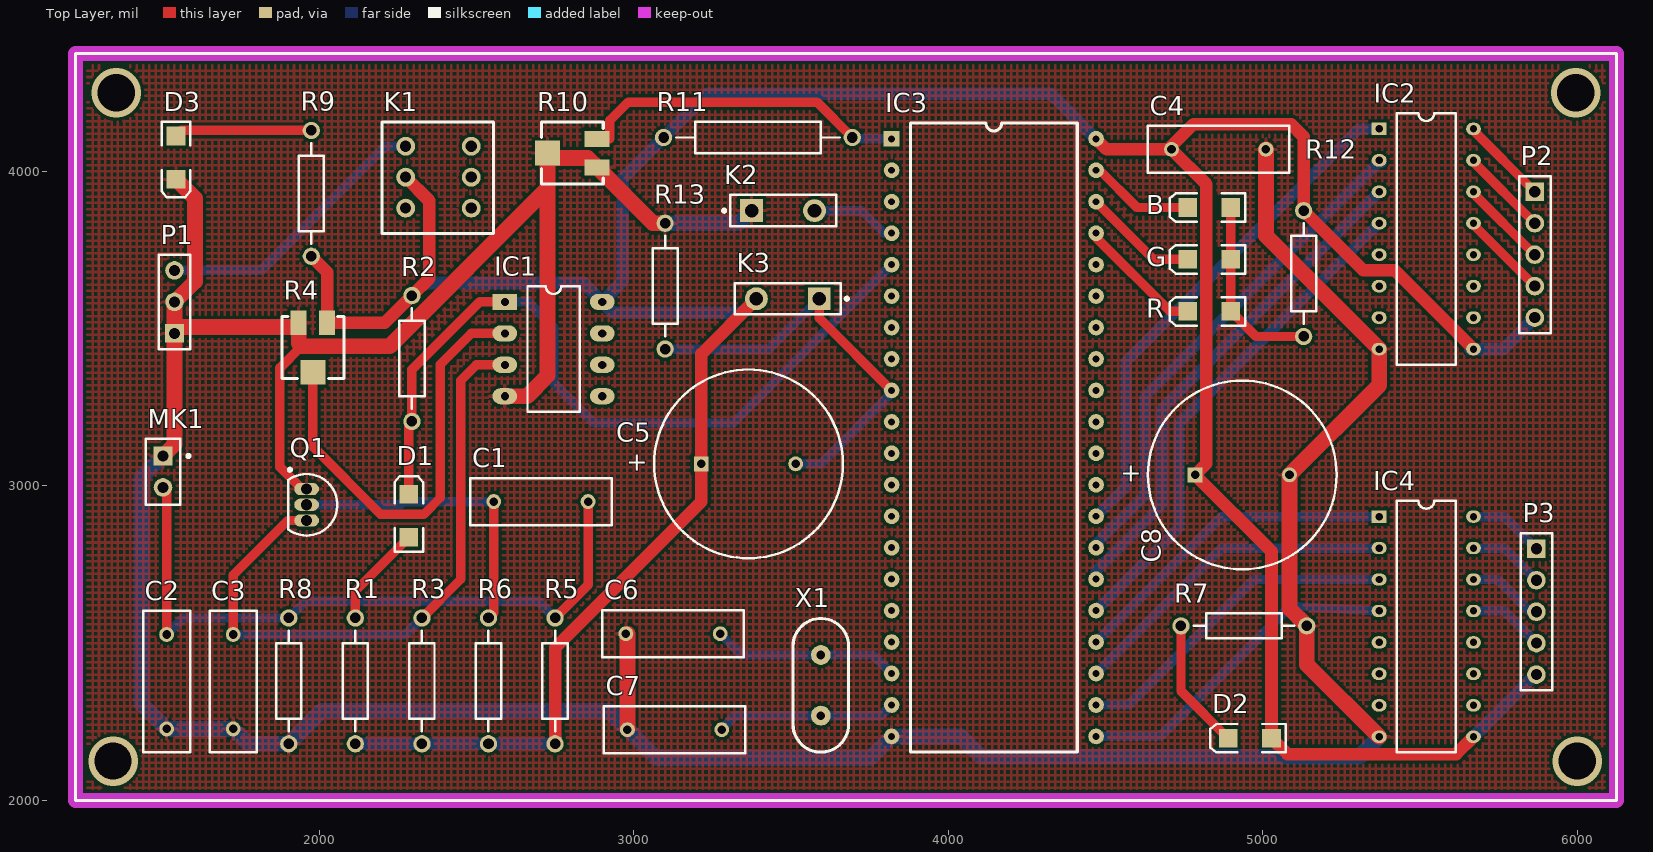
[diagram p0: Top Layer view]
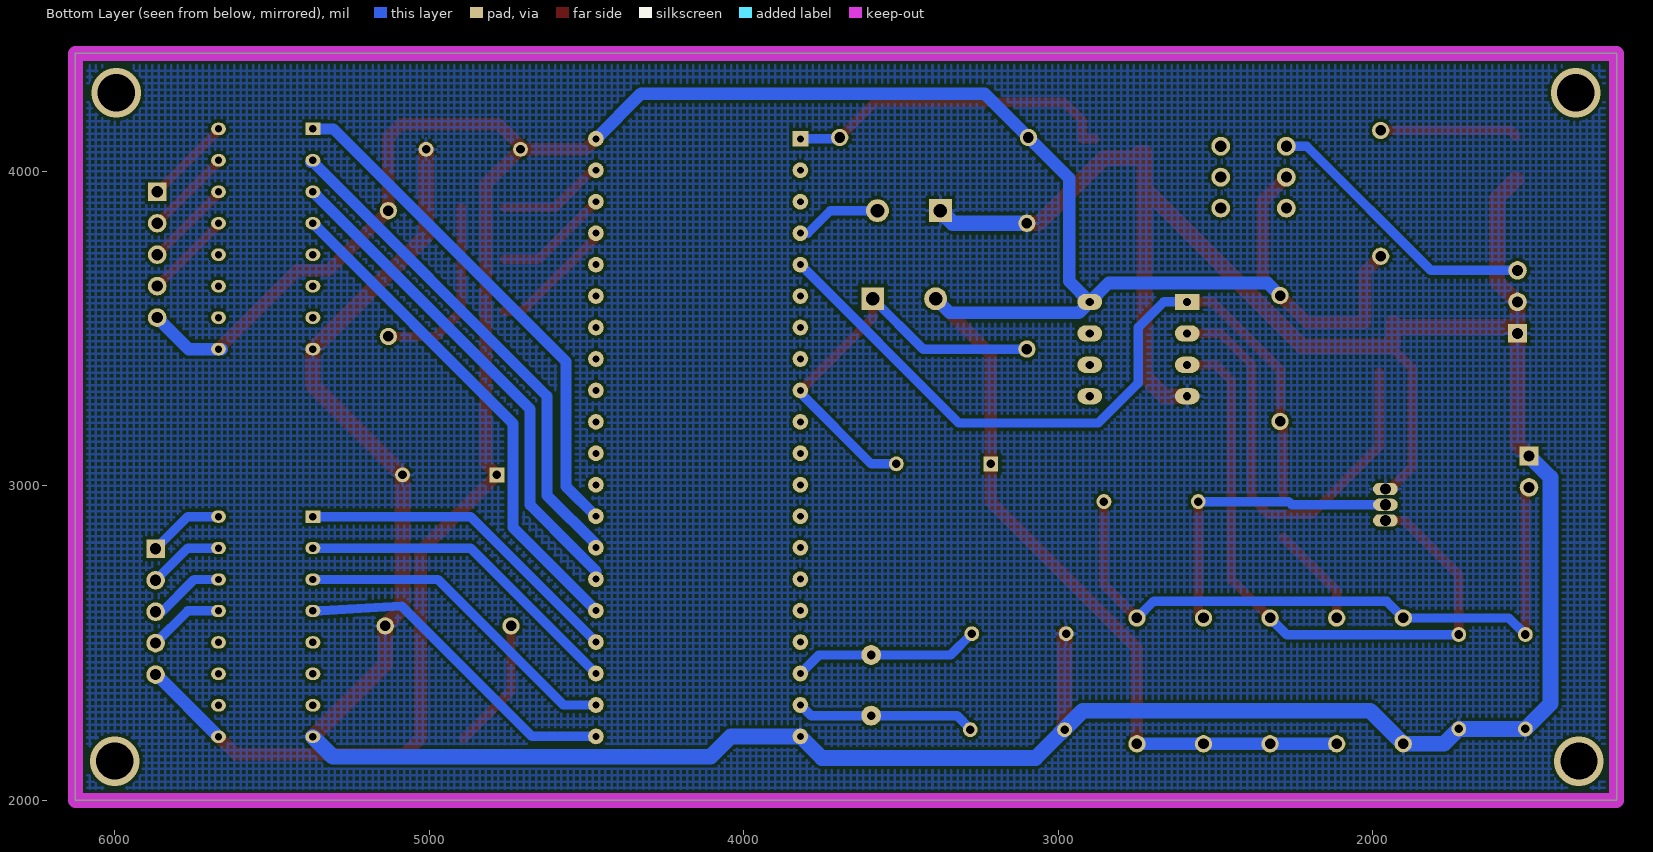
[diagram p1: Bottom Layer view, seen from below]
# Altium PCB MISC86340.PcbDoc
Units mil, origin at the board's own origin, x right, y up, seen from the top; angles counter-clockwise.
Board outline 4900 x 2375 mil, 2 copper layers (Top Layer, Bottom Layer); 40 components, 36 nets, 166 pads, 4 vias.

## Layer stack, top to bottom (the 12.6 mil dielectric is the usual default, probably not edited)
Top Solder: solder mask 0.4, Solder Resist, Dk 3.5
Top Layer: signal copper 1.4
Dielectric 1: dielectric 12.6, FR-4, Dk 4.8
Bottom Layer: signal copper 1.4
Bottom Solder: solder mask 0.4, Solder Resist, Dk 3.5

## Board outline
1225,2000 1225,4375 6125,4375 6125,2000

## Design rules (kind name [scope] priority, off if disabled: settings)
Clearance [All] p1: gap=10
HoleSize [All] p1: absolutevalues=TRUE maxlimit=500 minlimit=1 maxpercent=80.000 minpercent=20.000
MinimumSolderMaskSliver [All] p1: minsoldermaskwidth=2
PolygonConnect [All] p1: connectstyle=Relief reliefconductorwidth=10 reliefentries=4 polygonreliefangle="90 Angle" airgapwidth=10
RoomDefinition 声光控窗帘 [InComponentClass('声光控窗帘')] p1: confinementstyle=ConfineIn formatcopy=TRUE lockcomponents=FALSE outline 1205,1975 6145,1975 6145,4380 1205,4380
RoutingVias [All] p1: holewidth=28 width=50 viastyle="Through Hole" minholewidth=28 minwidth=50 maxholewidth=28 maxwidth=50
SilkToSilkClearance [All] p1: silktosilkclearance=2
SilkToSolderMaskClearance [IsPad] p1: minsilkscreentomaskgap=0 clearancetoexposedcopper=TRUE
SolderMaskExpansion [All] p1: expansion=4
Width GND [InNet('GND')] p1: maxlimit=55 minlimit=30 preferedwidth=50
Width VCC [InNet('VCC')] p2: maxlimit=45 minlimit=30 preferedwidth=40
Width [All] p3: maxlimit=35 minlimit=20 preferedwidth=30
26 further rules are at their usual default settings.

## Components (designator, comment, footprint, x,y, rotation, side; value= is the part's Value field where it differs from the comment)
B "LED2" 3.2X1.6X1.1 4830,3885 r180 top
C1 "Cap" RAD-0.3 2705,2950 r180 top
C2 "Cap" RAD-0.3 1515,2377.38 r270 top
C3 "Cap" RAD-0.3 1726.67,2377.38 r270 top
C4 "Cap" RAD-0.3 4860,4070 r0 top
C5 "Cap Pol1" RB7.6-15 3365,3070 r180 top
C6 "Cap" RAD-0.3 3125,2530 r180 top
C7 "Cap" RAD-0.3 3130,2225 r180 top
C8 "Cap Pol1" RB7.6-15 4935,3035 r180 top
D1 "LED2" 3.2X1.6X1.1 2285,2905 r90 top
D2 "LED2" 3.2X1.6X1.1 4958.9,2197.65 r180 top
D3 "LED2" 3.2X1.6X1.1 1544.72,4043.45 r270 top
G "LED2" 3.2X1.6X1.1 4830,3720 r180 top
IC1 "LM393" LM393 2590.16,3585 r0 top
IC2 "ULN2003" ULN2003 5370,4135 r0 top
IC3 "89c51" 89c51 3820,4103.44 r0 top
IC4 "ULN2003" ULN2003 5370,2902.38 r0 top
K1 "Component_1" 自锁开关 2200,4156.56 r270 top
K2 "SW-PB" SPST-2 3475,3875 r0 top
K3 "SW-PB" SPST-2 3490,3595 r180 top
MK1 "Mic2" PIN2 1503.39,3095 r270 top
P1 "Header 3" HDR1X3 1540,3485 r90 top
P2 "Header 5" HDR1X5 5865,3935 r270 top
P3 "Header 5" HDR1X5 5870,2800 r270 top
Q1 "2N3904" TO-92A 1960,2940 r180 top
R "LED2" 3.2X1.6X1.1 4830,3555 r180 top
R1 "Res2" AXIAL-0.4 2115,2380 r90 top
R2 "Res2" AXIAL-0.4 2295,3405 r270 top
R3 "Res2" AXIAL-0.4 2326.67,2380 r270 top
R4 "RPot SM" POT4MM-2 1980,3440 r270 top
R5 "Res2" AXIAL-0.4 2750,2380 r270 top
R6 "Res2" AXIAL-0.4 2538.33,2380 r270 top
R7 "Res2" AXIAL-0.4 4940,2555 r180 top
R8 "Res2" AXIAL-0.4 1903.33,2380 r90 top
R9 "Res2" AXIAL-0.4 1975,3930 r90 top
R10 "RPot SM" POT4MM-2 2805,4058.13 r180 top
R11 "Res Adj2" AXIAL-0.6 3395,4107.62 r180 top
R12 "Res2" AXIAL-0.4 5130,3675 r270 top
R13 "Res2" AXIAL-0.4 3100,3635 r90 top
X1 "Component_1" LC-HC-49S 3595,2365.94 r90 top

## Footprints (in the part's own frame and the unit in brackets; to place one, negate y for a bottom-side part, rotate by r counter-clockwise, add the part's x,y. Pads: shape width x height; smd on the part's side, far side on the other; paste and mask are expansions set on the pad)
3.2X1.6X1.1 [mm] "SMT LED; 2 Flat Leads"
  rect 1.5x1.5 smd: 1(-1.75,0) 2(1.75,0)
  silkscreen extent -2.9,-1.15 3.2,1.15
89c51 [mil]
  rect 50x50 hole 22: 1(0,0)
  round 50 hole 22: 2(0,-100) 3(0,-200) 4(0,-300) 5(0,-400) 6(0,-500) 7(0,-600) 8(0,-700) 9(0,-800) 10(0,-900) 11(0,-1000) 12(0,-1100) 13(0,-1200) 14(0,-1300) 15(0,-1400) 16(0,-1500) 17(0,-1600) 18(0,-1700) 19(0,-1800) 20(0,-1900) 21(650,-1900) 22(650,-1800) 23(650,-1700) 24(650,-1600) 25(650,-1500) 26(650,-1400) 27(650,-1300) 28(650,-1200) 29(650,-1100) 30(650,-1000) 31(650,-900) 32(650,-800) 33(650,-700) 34(650,-600) 35(650,-500) 36(650,-400) 37(650,-300) 38(650,-200) 39(650,-100) 40(650,0)
  silkscreen extent 60,-1950 590,50, body extent 65,-1950 590,55, height 190
AXIAL-0.4 [mm] "Axial Device, Thru-Hole; 2 Leads; 0.4 in Pin Spacing"
  round 1.4 hole 0.85: 1(-5.08,0) 2(5.08,0)
  silkscreen extent -4.06,-1.02 4.06,1.02
AXIAL-0.6 [mm] "Axial Device, Thru-Hole; 2 Leads; 0.6 in Pin Spacing"
  round 1.4 hole 0.85: 1(-7.62,0) 2(7.62,0)
  silkscreen extent -6.6,-1.27 6.6,1.27
HDR1X3 [mm] "Connector; Header; 3 Position"
  rect 1.5x1.5 hole 0.9: 1(0,0)
  round 1.5 hole 0.9: 2(2.54,0) 3(5.08,0)
  silkscreen extent -1.27,-1.27 6.35,1.27
HDR1X5 [mm] "Connector; Header; 5 Position"
  rect 1.5x1.5 hole 0.9: 1(0,0)
  round 1.5 hole 0.9: 2(2.54,0) 3(5.08,0) 4(7.62,0) 5(10.16,0)
  silkscreen extent -1.27,-1.27 11.43,1.27
LC-HC-49S [mm]
  round 1.6 hole 0.7: 1(-2.45,0) 2(2.45,0)
  silkscreen extent -5.39,-2.25 5.39,2.25
LM393 [mm]
  rect 2x1.3 hole 0.65: 1(0,0)
  oval 2x1.3 hole 0.65: 2(0,-2.54) 3(0,-5.08) 4(0,-7.62) 5(7.87,-7.62) 6(7.87,-5.08) 7(7.87,-2.54) 8(7.87,0)
  silkscreen extent 1.84,-8.89 6.04,1.27
PIN2 [mm] "Photosensitive Diode; 2 Leads"
  rect 1.5x1.5 hole 0.9: 1(0,0)
  round 1.5 hole 0.9: 2(2.54,0)
  silkscreen extent -1.4,-1.4 3.94,2.18
POT4MM-2 [mm] "Square Trimming Potentiometer"
  rect 2x1.3 smd: CCW(-2,-1.15) CW(-2,1.15)
  rect 2x2 smd: W(2,0)
  silkscreen extent -2.5,-2.5 2.5,2.5
RAD-0.3 [mm] "Radial Cap, Thru-Hole; 2 Leads; 0.3 in Pin Spacing"
  round 1.2 hole 0.7: 1(-3.81,0) 2(3.81,0)
  silkscreen extent -5.71,-1.91 5.71,1.91
RB7.6-15 [mm] "Polarized Capacitor (Radial); 2 Leads"
  rect 1.2x1.2 hole 0.7: 1(3.81,0)
  round 1.2 hole 0.7: 2(-3.81,0)
  silkscreen extent -7.62,-7.62 7.62,7.62
SPST-2 [mm] "Switch; 2 Leads"
  rect 1.85x1.85 hole 1.1: 1(-2.54,0)
  round 1.85 hole 1.1: 2(2.54,0)
  silkscreen extent -4.89,-1.27 4.28,1.27
TO-92A [mm] "TO, Flat Index; 3 In-Line, Axial Leads; Body Dia. 4.5mm; Leads 0.51 x 0.48 mm (max)"
  oval 2x1 hole 0.9: 1(0,-1.27) 2(0,0) 3(0,1.27)
  silkscreen extent -2.48,-2.95 1.5,2.48, body extent -2.48,-2.5 1.5,2.5, height 6.86
ULN2003 [mm]
  rect 1.2x1 hole 0.6: 1(0,0)
  oval 1.2x1 hole 0.6: 2(0,-2.54) 3(0,-5.08) 4(0,-7.62) 5(0,-10.16) 6(0,-12.7) 7(0,-15.24) 8(0,-17.78) 9(7.62,-17.78) 10(7.62,-15.24) 11(7.62,-12.7) 12(7.62,-10.16) 13(7.62,-7.62) 14(7.62,-5.08) 15(7.62,-2.54) 16(7.62,0)
  silkscreen extent 1.43,-19.05 6.19,1.27
自锁开关 [mil]
  round 60 hole 35.43: 1(76.58,75) 2(175,75) 3(273.43,75) 4(76.58,283.66) 5(175,283.66) 6(273.43,283.66)
  silkscreen extent 0,0 354,354

## Part data
B D1 D2 D3 G R: "Typical RED, GREEN, YELLOW, AMBER GaAs LED"
C1 C2 C3 C4 C6 C7: "Capacitor"
C5 C8: "Polarized Capacitor (Radial)"
IC1 IC2 IC3 IC4: library part Component_1
K2 K3: "Switch"
MK1: "Microphone"
P1: "Header, 3-Pin"
P2 P3: "Header, 5-Pin"
Q1: "NPN General Purpose Amplifier"
R1 R2 R3 R5 R6 R7 R8 R9 R12 R13: "Resistor"
R4 R10: "Square Trimming Potentiometer"
R11: "Variable Resistor"

## Via types
v1: diameter 157.48, hole 118.11, Top Layer to Bottom Layer, 4 vias

## Nets (pads, with @x,y where several pads share a name; then routed paths per layer and width w, separated by ;. In a path a pad name is that pad's centre, name@x,y a point inside that pad or via, vN(x,y) a via of type N, cw(c..) or ccw(c..) an arc to the next point about the centre after c; other vN are vias at no path point)
GND: C2.2 C3.2 C4.2 C6.2 C7.2 C8.2 D3.2 IC1.4 IC2.8 IC3.20 IC4.8 K2.1 MK1.1 P1.1 P1.2 Q1.1 R4.CCW R7.1 R8.1 R10.CW R10.W R13.2 | length 12125.8
  Top Layer w30: 1944,3444 1875,3375 1875,3060 1945,2990 Q1.1
  Top Layer w50: MK1.1 1540,3131.61 P1.1 ; D3.2 1605,3914.28 1605,3650 P1.2 P1.1 ; IC1.4 2661.26,3285 2726.26,3350 2726.26,3946.26 ; C7.2@2980,2227.38 C6.2@2980,2530 ; R13.2 3061.6,3835 R10.CW 2853.78,4042.82 2757.18,4042.82 2741.87,4058.13 R10.W 2726.26,3946.26 ; C4.2 5010,3795 IC2.8 5370,3320 C8.2 5085,2610 R7.1 5140,2432.38 IC4.8 ; P1.1 1560,3505 1920.98,3505 R4.CCW 1934.72,3453.28 1944,3444 2224,3444 2726.26,3946.26
  Bottom Layer w50: MK1.1 1435,3026.61 1435,2307.38 C2.2 C3.2 1774.04,2180 R8.1 2008.33,2285 2922.38,2285 3072.38,2135 3751.56,2135 IC3.20 4041.56,2203.44 4106,2139 5306.62,2139 IC4.8 ; R13.2 3335,3835 K2.1
NetB_1: B.1 G.1 R12.2 R.1 | length 594.2
  Top Layer w30: B.1 G.1 R.1 4978.9,3475 R12.2
NetB_2: B.2 IC3.39 | length 340.2
  Top Layer w30: IC3.39 4481.56,4003.44 4600,3885 B.2
NetC1_1: C1.1 C2.1 MK1.2 R5.1 R8.2 | length 2186.6
  Top Layer w30: MK1.2 1515,2983.39 C2.1 ; R5.1 2855,2685 C1.1
  Bottom Layer w30: C2.1 1567.62,2580 R8.2 1956.33,2633 2697,2633 R5.1
NetC1_2: C1.2 Q1.2 R6.1 | length 976
  Top Layer w30: R6.1 2555,2596.67 C1.2
  Bottom Layer w30: Q1.2 2258,2940 2268,2950 C1.2
NetC3_1: C3.1 IC1.3 Q1.3 R3.1 | length 2083.2
  Top Layer w30: C3.1 1726.67,2716.67 1900,2890 Q1.3 ; R3.1 2450,2703.33 2450,3335 2500,3385 IC1.3
  Bottom Layer w30: C3.1 2274.04,2527.38 R3.1
NetC5_2: C5.2 IC3.9 K3.1 R13.1 | length 1349.7
  Top Layer w30: K3.1 3590,3533.44 IC3.9
  Bottom Layer w30: R13.1 3430,3435 K3.1 ; C5.2 3595,3070 3820,3295 IC3.9
NetC6_1: C6.1 IC3.18 X1.2 | length 597.4
  Bottom Layer w30: C6.1 3342.6,2462.4 X1.2 3761.04,2462.4 IC3.18
NetC7_1: C7.1 IC3.19 X1.1 | length 571.5
  Bottom Layer w30: C7.1@3280,2227.38 3322.11,2269.48 X1.1 3786.04,2269.48 IC3.19
NetD1_1: D1.1 R1.2 | length 326.5
  Top Layer w30: R1.2 2115,2666.1 D1.1
NetD2_2: D2.2 R7.2 | length 419.5
  Top Layer w30: R7.2 4740,2347.65 D2.2
NetD3_1: D3.1 R9.2 | length 437.6
  Top Layer w30: D3.1 1562.38,4130 R9.2
NetG_2: G.2 IC3.38 | length 367.1
  Top Layer w30: IC3.38 4653.44,3720 G.2
NetIC1_2: IC1.2 R4.W | length 1422
  Top Layer w30: R4.W 1980,3125 2195,2910 2333,2910 2385,2962 2385,3386 2484,3485 IC1.2
NetIC2_13: IC2.13 P2.4 | length 280.8
  Top Layer w30: IC2.13 5670,3830 P2.4
NetIC2_14: IC2.14 P2.3 | length 280.8
  Top Layer w30: IC2.14 5670,3930 P2.3
NetIC2_15: IC2.15 P2.2 | length 280.8
  Top Layer w30: IC2.15 5670,4030 P2.2
NetIC2_16: IC2.16 P2.1 | length 280.8
  Top Layer w30: IC2.16 5670,4130 P2.1
NetIC3_4: IC3.4 K2.2 | length 274.6
  Bottom Layer w30: K2.2 3725,3875 3796.56,3803.44 IC3.4
NetIC3_37: IC3.37 R.2 | length 401.9
  Top Layer w30: IC3.37 4470,3790 4705,3555 R.2
NetIC4_13: IC4.13 P3.4 | length 242.4
  Bottom Layer w30: IC4.13 5767.62,2602.38 P3.4
NetIC4_14: IC4.14 P3.3 | length 242.4
  Bottom Layer w30: IC4.14 5747.62,2702.38 5850,2600 P3.3
NetIC4_15: IC4.15 P3.2 | length 242.4
  Bottom Layer w30: IC4.15 5767.62,2802.38 P3.2
NetIC4_16: IC4.16 P3.1 | length 242.4
  Bottom Layer w30: IC4.16 5767.62,2902.38 P3.1
NetK1_1: K1.1 P1.3 | length 898.6
  Bottom Layer w30: P1.3 1815,3685 2209.98,4079.98 K1.1
P1.0: IC3.1 R10.CCW R11.1 | length 1067.2
  Top Layer w30: R10.CCW 2924.06,4103.41 2924.06,4161.8 2982.44,4220.18 3582.44,4220.18 R11.1
  Bottom Layer w30: R11.1 3699.18,4103.44 IC3.1
P1.4: D1.2 IC1.1 IC3.5 R2.2 | length 2486
  Top Layer w30: D1.2 2285,3195 R2.2 2295,3370 2510,3585 IC1.1
  Bottom Layer w30: IC1.1 2665,3585 2746,3504 2746,3327 2873,3200 3316.56,3200 IC3.5
P2.0: IC3.21 IC4.4 | length 1072.2
  Bottom Layer w30: IC3.21 4673.44,2203.44 5088,2618 5344,2602.38 IC4.4
P2.1: IC3.22 IC4.3 | length 1065.2
  Bottom Layer w30: IC3.22 4573.44,2303.44 4972.38,2702.38 IC4.3
P2.2: IC3.23 IC4.2 | length 1065.2
  Bottom Layer w30: IC3.23 4868.94,2802.38 IC4.2
P2.3: IC3.24 IC4.1 | length 1065.2
  Bottom Layer w30: IC3.24 4868.94,2902.38 IC4.1
P2.4: IC2.4 IC3.25 | length 1604.4
  Bottom Layer w35: IC3.25 4733.88,2867.32 4733.88,3198.88 IC2.4
P2.5: IC2.3 IC3.26 | length 1604.1
  Bottom Layer w35: IC3.26 4470,2729.2 4530.4,2789.6 ; 4530,2790 4680,2940 4680,3245 IC2.3
P2.6: IC2.2 IC3.27 | length 1605.8
  Bottom Layer w35: IC3.27 4470,2815 4625,2970 4625,3285 5367.5,4027.5 IC2.2@5377.5,4027.5
P2.7: IC2.1 IC3.28 | length 1642.4
  Bottom Layer w35: IC3.28 4565,2998.44 4565,3395 5305,4135 IC2.1
VCC: C4.1 C5.1 C8.1 D2.1 IC1.8 IC2.9 IC3.40 IC4.9 K1.2 K3.2 P2.5 P3.5 R1.1 R2.1 R3.2 R4.CW R5.2 R6.2 R9.1 R11.2 R12.1 | length 11482.8
  Top Layer w40: R9.1 2025.28,3679.72 R4.CW 2208.74,3518.74 R2.1 2350,3660 2350,3906.56 K1.2 ; R5.2 2750,2485 3215,2950 C5.1 3215,3420 K3.2 ; IC3.40 4503.44,4070 C4.1 ; IC4.9 5615,2147.38 5078.07,2147.38 D2.1 5027.8,2792.2 C8.1 4821,3071 4821,3959 C4.1 ; IC2.9 5420,3685 5320,3685 R12.1 5130,4110 5090,4150 4780,4150 4710,4080 C4.1
  Bottom Layer w40: R1.1 R3.2 R6.2 R5.2 ; R2.1 2335,3645 2840,3645 IC1.8 ; K3.2 3345,3550 2935,3550 IC1.8 ; IC3.40 4326.44,4247 3234.38,4247 R11.2 2965,3977.62 2965,3650 IC1.8 ; IC2.9@5660,3435 IC2.9 5765,3435 P2.5 ; IC4.9 5867.62,2400 P3.5
pads on no net: IC1.5 IC1.6 IC1.7 IC2.5 IC2.6 IC2.7 IC2.10 IC2.11 IC2.12 IC3.2 IC3.3 IC3.6 IC3.7 IC3.8 IC3.10 IC3.11 IC3.12 IC3.13 IC3.14 IC3.15 IC3.16 IC3.17 IC3.29 IC3.30 IC3.31 IC3.32 IC3.33 IC3.34 IC3.35 IC3.36 IC4.5 IC4.6 IC4.7 IC4.10 IC4.11 IC4.12 K1.3 K1.4 K1.5 K1.6
copper on no net:
  other v1: 1345,2125 6000,2125 1355,4250 5995,4250

## Polygon pours and split planes (outlines as drawn)
GND on Top Layer "Top Layer-No Net" (hatched 90Degree grid 20 track 8, pour order 2): 1225,2000 6125,2000 6115,2010 6115,4375 1225,4375
GND on Bottom Layer "Top Layer-No Net" (hatched 90Degree grid 20 track 8, pour order 4): 1225,4375 6105,4375 6105,2020 6125,2000 1225,2000

## Keep-outs
Keep-Out Layer:
  the board outline again, w47.24

## Silkscreen, mask and mechanical layers (free items; w line width, h text height)
Top Overlay:
  lines w10: 1225,2000 1225,4375 1250,4375 6125,4375 6125,2000 1225,2000